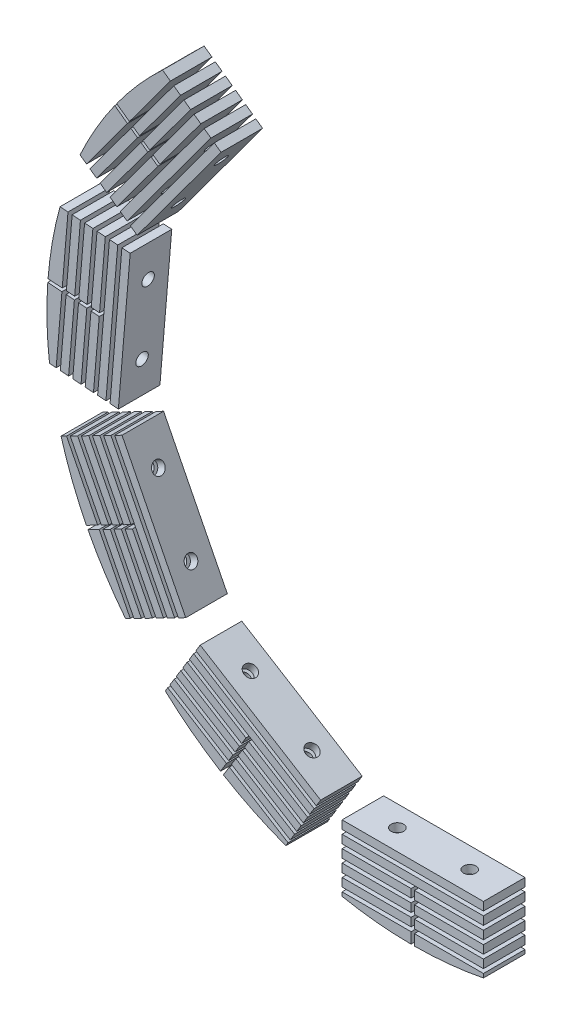
SolidWorks part; units mm, degrees
ref_plane "前视基准面" through (0, 0, 0) normal (0, 0, 1) x (1, 0, 0)
ref_plane "上视基准面" through (0, 0, 0) normal (0, 1, 0) x (1, 0, 0)
ref_plane "右视基准面" through (0, 0, 0) normal (1, 0, 0) x (0, 0, -1)
other "Configuration Table"
sketch "草图1" plane through (0, 0, 0) normal (0, 0, 1) x (1, 0, 0)
  line L0 (-85, -337) -> (-85, -431.7117)
  line L1 (-85, -337) -> (85, -337)
  line L5 (85, -337) -> (85, -431.7117)
  line L18 (-266.8501, -222.677) -> (-129.3172, -322.6005)
  line L19 (-266.8501, -222.677) -> (-322.5202, -299.3004)
  line L20 (-129.3172, -322.6005) -> (-184.9873, -399.2239)
  line L21 (-346.7725, -23.2989) -> (-294.2396, -184.9785)
  line L22 (-346.7725, -23.2989) -> (-436.8487, -52.5665)
  line L23 (-294.2396, -184.9785) -> (-384.3158, -214.2461)
  line L24 (-294.2396, 184.9785) -> (-346.7725, 23.2989)
  line L25 (-294.2396, 184.9785) -> (-384.3158, 214.2461)
  line L26 (-346.7725, 23.2989) -> (-436.8487, 52.5665)
  line L27 (-129.3172, 322.6005) -> (-266.8501, 222.677)
  line L28 (-129.3172, 322.6005) -> (-184.9873, 399.2239)
  line L29 (-266.8501, 222.677) -> (-322.5202, 299.3004)
  line L30 (85, 337) -> (-85, 337)
  line L31 (85, 337) -> (85, 431.7117)
  line L32 (-85, 337) -> (-85, 431.7117)
  line L33 (266.8501, 222.677) -> (129.3172, 322.6005)
  line L34 (266.8501, 222.677) -> (322.5202, 299.3004)
  line L35 (129.3172, 322.6005) -> (184.9873, 399.2239)
  line L36 (346.7725, 23.2989) -> (294.2396, 184.9785)
  line L37 (346.7725, 23.2989) -> (436.8487, 52.5665)
  line L38 (294.2396, 184.9785) -> (384.3158, 214.2461)
  line L39 (294.2396, -184.9785) -> (346.7725, -23.2989)
  line L40 (294.2396, -184.9785) -> (384.3158, -214.2461)
  line L41 (346.7725, -23.2989) -> (436.8487, -52.5665)
  line L42 (129.3172, -322.6005) -> (266.8501, -222.677)
  line L43 (129.3172, -322.6005) -> (184.9873, -399.2239)
  line L44 (266.8501, -222.677) -> (322.5202, -299.3004)
  arc A2 (-85, -431.7117) -> (85, -431.7117) centre (0, 0) ccw
  arc A5 (-322.5202, -299.3004) -> (-184.9873, -399.2239) centre (0, 0) ccw
  arc A6 (-436.8487, -52.5665) -> (-384.3158, -214.2461) centre (0, 0) ccw
  arc A7 (-384.3158, 214.2461) -> (-436.8487, 52.5665) centre (0, 0) ccw
  arc A8 (-184.9873, 399.2239) -> (-322.5202, 299.3004) centre (0, 0) ccw
  arc A9 (85, 431.7117) -> (-85, 431.7117) centre (0, 0) ccw
  arc A10 (322.5202, 299.3004) -> (184.9873, 399.2239) centre (0, 0) ccw
  arc A11 (436.8487, 52.5665) -> (384.3158, 214.2461) centre (0, 0) ccw
  arc A12 (384.3158, -214.2461) -> (436.8487, -52.5665) centre (0, 0) ccw
  arc A13 (184.9873, -399.2239) -> (322.5202, -299.3004) centre (0, 0) ccw
  point P7 (0, -337)
  dimension "D1" = 440
  dimension "D2" = 337
  dimension "D3" = 170
  dimension "D4" = 10
sketch "草图2" plane through (0, 0, 0) normal (0, 0, 1) x (1, 0, 0)
  line L0 (-85, -337) -> (-85, -431.7117)
  line L1 (-85, -337) -> (85, -337) construction
  line L2 (85, -337) -> (85, -431.7117)
  line L3 (0, -299.5672) -> (0, -474.8241) construction
  line L4 (-85, -337) -> (-2, -337)
  line L5 (-2, -337) -> (-2, -439.9955)
  line L6 (2, -337) -> (2, -439.9955)
  line L7 (85, -337) -> (2, -337)
  line L8 (-248.2534, -243.237) -> (-177.4302, -286.5162)
  line L9 (-248.2534, -243.237) -> (-297.6394, -324.0537)
  line L10 (-177.4302, -286.5162) -> (-231.1357, -374.4012)
  line L11 (-174.0171, -288.6019) -> (-227.7225, -376.487)
  line L12 (-103.1939, -331.881) -> (-174.0171, -288.6019)
  line L13 (-103.1939, -331.881) -> (-152.58, -412.6977)
  line L14 (-338.6647, -78.1039) -> (-300.7992, -151.9632)
  line L15 (-338.6647, -78.1039) -> (-422.946, -121.3124)
  line L16 (-300.7992, -151.9632) -> (-392.452, -198.9509)
  line L17 (-298.9744, -155.5227) -> (-390.6271, -202.5104)
  line L18 (-261.1089, -229.3821) -> (-298.9744, -155.5227)
  line L19 (-261.1089, -229.3821) -> (-345.3902, -272.5906)
  line L20 (-329.7056, 109.9464) -> (-335.9082, 27.1784)
  line L21 (-329.7056, 109.9464) -> (-424.1525, 117.0242)
  line L22 (-335.9082, 27.1784) -> (-438.6157, 34.8753)
  line L23 (-336.2071, 23.1896) -> (-438.9146, 30.8865)
  line L24 (-342.4097, -59.5783) -> (-336.2071, 23.1896)
  line L25 (-342.4097, -59.5783) -> (-436.8566, -52.5005)
  line L26 (-224.0049, 265.7363) -> (-272.4556, 198.3455)
  line L27 (-224.0049, 265.7363) -> (-300.9049, 321.0237)
  line L28 (-272.4556, 198.3455) -> (-356.0815, 258.4684)
  line L29 (-274.7906, 195.0977) -> (-358.4165, 255.2207)
  line L30 (-323.2413, 127.7069) -> (-274.7906, 195.0977)
  line L31 (-323.2413, 127.7069) -> (-400.1414, 182.9942)
  arc A0 (-85, -431.7117) -> (85, -431.7117) centre (0, 0) ccw construction
  arc A1 (-85, -431.7117) -> (-2, -439.9955) centre (0, 0) ccw
  arc A2 (85, -431.7117) -> (2, -439.9955) centre (0, 0) cw
  arc A3 (-297.6394, -324.0537) -> (-231.1357, -374.4012) centre (0, 0) ccw
  arc A4 (-152.58, -412.6977) -> (-227.7225, -376.487) centre (0, 0) cw
  arc A5 (-422.946, -121.3124) -> (-392.452, -198.9509) centre (0, 0) ccw
  arc A6 (-345.3902, -272.5906) -> (-390.6271, -202.5104) centre (0, 0) cw
  arc A7 (-424.1525, 117.0242) -> (-438.6157, 34.8753) centre (0, 0) ccw
  arc A8 (-436.8566, -52.5005) -> (-438.9146, 30.8865) centre (0, 0) cw
  arc A9 (-300.9049, 321.0237) -> (-356.0815, 258.4684) centre (0, 0) ccw
  arc A10 (-400.1414, 182.9942) -> (-358.4165, 255.2207) centre (0, 0) cw
  point P2 (0, -387.1957)
  dimension "D1" = 2
  dimension "D3" = 31.429
  dimension "D2" = 5
extrude "凸台-拉伸1" add sketch "草图2" along normal mid plane 50
sketch "草图3" plane through (0, 0, 25) normal (0, 0, 1) x (1, 0, 0)
  line L0 (85, -337) -> (2, -337) construction
  line L1 (-88.6131, -347) -> (106.3869, -347)
  line L2 (-88.6131, -347) -> (-88.6131, -352)
  line L3 (-88.6131, -352) -> (106.3869, -352)
  line L4 (106.3869, -347) -> (106.3869, -352)
  line L5 (-88.6131, -362) -> (106.3869, -362)
  line L6 (-88.6131, -367) -> (106.3869, -367)
  line L7 (-88.6131, -362) -> (-88.6131, -367)
  line L8 (106.3869, -362) -> (106.3869, -367)
  line L9 (-88.6131, -377) -> (106.3869, -377)
  line L10 (-88.6131, -382) -> (106.3869, -382)
  line L11 (-88.6131, -377) -> (-88.6131, -382)
  line L12 (106.3869, -377) -> (106.3869, -382)
  line L13 (-88.6131, -392) -> (106.3869, -392)
  line L14 (-88.6131, -397) -> (106.3869, -397)
  line L15 (-88.6131, -392) -> (-88.6131, -397)
  line L16 (106.3869, -392) -> (106.3869, -397)
  line L17 (-88.6131, -407) -> (106.3869, -407)
  line L18 (-88.6131, -412) -> (106.3869, -412)
  line L19 (-88.6131, -407) -> (-88.6131, -412)
  line L20 (106.3869, -407) -> (106.3869, -412)
  line L21 (-88.6131, -422) -> (106.3869, -422)
  line L22 (-88.6131, -427) -> (106.3869, -427)
  line L23 (-88.6131, -422) -> (-88.6131, -427)
  line L24 (106.3869, -422) -> (106.3869, -427)
  line L231 (-297.2911, -317.7031) -> (-131.2044, -419.8803)
  line L242 (-347.3723, -74.3518) -> (-351.8663, -76.5436) [skipped]
  line L243 (-360.8542, -80.9274) -> (-365.3482, -83.1192) [skipped]
  line L244 (-374.3361, -87.5029) -> (-378.8301, -89.6948) [skipped]
  line L245 (-387.818, -94.0785) -> (-392.312, -96.2703) [skipped]
  line L246 (-401.2999, -100.6541) -> (-405.7939, -102.8459) [skipped]
  line L247 (-414.7819, -107.2296) -> (-419.2758, -109.4215) [skipped]
  line L248 (-332.0417, 120.5654) -> (-352.4248, -73.3664) [skipped]
  line L249 (-332.0417, 120.5654) -> (-337.0143, 121.088) [skipped]
  line L250 (-337.0143, 121.088) -> (-357.3974, -72.8437) [skipped]
  line L251 (-352.4248, -73.3664) -> (-357.3974, -72.8437) [skipped]
  line L252 (-367.3426, -71.7984) -> (-372.3152, -71.2758) [skipped]
  line L253 (-382.2604, -70.2305) -> (-387.233, -69.7079) [skipped]
  line L254 (-397.1783, -68.6626) -> (-402.1509, -68.14) [skipped]
  line L255 (-412.0961, -67.0947) -> (-417.0687, -66.572) [skipped]
  line L256 (-427.0139, -65.5267) -> (-431.9865, -65.0041) [skipped]
  line L257 (-346.9596, 122.1333) -> (-351.9322, 122.656) [skipped]
  line L258 (-361.8774, 123.7012) -> (-366.85, 124.2239) [skipped]
  line L259 (-376.7952, 125.2692) -> (-381.7678, 125.7918) [skipped]
  line L260 (-391.713, 126.8371) -> (-396.6856, 127.3597) [skipped]
  line L261 (-406.6309, 128.405) -> (-411.6035, 128.9277) [skipped]
  line L262 (-346.9596, 122.1333) -> (-367.3426, -71.7984) [skipped]
  line L263 (-351.9322, 122.656) -> (-372.3152, -71.2758) [skipped]
  line L264 (-361.8774, 123.7012) -> (-382.2604, -70.2305) [skipped]
  line L265 (-366.85, 124.2239) -> (-387.233, -69.7079) [skipped]
  line L266 (-376.7952, 125.2692) -> (-397.1783, -68.6626) [skipped]
  line L267 (-381.7678, 125.7918) -> (-402.1509, -68.14) [skipped]
  line L268 (-391.713, 126.8371) -> (-412.0961, -67.0947) [skipped]
  line L269 (-396.6856, 127.3597) -> (-417.0687, -66.572) [skipped]
  line L270 (-406.6309, 128.405) -> (-427.0139, -65.5267) [skipped]
  line L271 (-411.6035, 128.9277) -> (-431.9865, -65.0041) [skipped]
  line L272 (-215.7503, 277.7406) -> (-335.8043, 124.0785) [skipped]
  line L273 (-215.7503, 277.7406) -> (-219.6903, 280.8189) [skipped]
  line L274 (-219.6903, 280.8189) -> (-339.7443, 127.1568) [skipped]
  line L275 (-335.8043, 124.0785) -> (-339.7443, 127.1568) [skipped]
  line L276 (-347.6244, 133.3134) -> (-351.5645, 136.3917) [skipped]
  line L277 (-359.4446, 142.5483) -> (-363.3847, 145.6266) [skipped]
  line L278 (-371.2648, 151.7832) -> (-375.2048, 154.8616) [skipped]
  line L279 (-383.0849, 161.0182) -> (-387.025, 164.0965) [skipped]
  line L280 (-394.9051, 170.2531) -> (-398.8451, 173.3314) [skipped]
  line L281 (-227.5705, 286.9755) -> (-231.5105, 290.0538) [skipped]
  line L282 (-239.3906, 296.2104) -> (-243.3307, 299.2887) [skipped]
  line L283 (-251.2108, 305.4453) -> (-255.1508, 308.5236) [skipped]
  line L284 (-263.0309, 314.6803) -> (-266.971, 317.7586) [skipped]
  line L285 (-274.8511, 323.9152) -> (-278.7912, 326.9935) [skipped]
  line L286 (-227.5705, 286.9755) -> (-347.6244, 133.3134) [skipped]
  line L287 (-231.5105, 290.0538) -> (-351.5645, 136.3917) [skipped]
  line L288 (-239.3906, 296.2104) -> (-359.4446, 142.5483) [skipped]
  line L289 (-243.3307, 299.2887) -> (-363.3847, 145.6266) [skipped]
  line L290 (-251.2108, 305.4453) -> (-371.2648, 151.7832) [skipped]
  line L291 (-255.1508, 308.5236) -> (-375.2048, 154.8616) [skipped]
  line L292 (-263.0309, 314.6803) -> (-383.0849, 161.0182) [skipped]
  line L293 (-266.971, 317.7586) -> (-387.025, 164.0965) [skipped]
  line L294 (-274.8511, 323.9152) -> (-394.9051, 170.2531) [skipped]
  line L295 (-278.7912, 326.9935) -> (-398.8451, 173.3314) [skipped]
  line L296 (-33.8394, 349.4076) -> (-217.0795, 282.7137) [skipped]
  line L297 (-33.8394, 349.4076) -> (-35.5495, 354.1061) [skipped]
  line L298 (-35.5495, 354.1061) -> (-218.7896, 287.4122) [skipped]
  line L299 (-217.0795, 282.7137) -> (-218.7896, 287.4122) [skipped]
  line L300 (-222.2098, 296.8091) -> (-223.9199, 301.5075) [skipped]
  line L301 (-227.3401, 310.9045) -> (-229.0502, 315.6029) [skipped]
  line L302 (-232.4704, 324.9999) -> (-234.1805, 329.6983) [skipped]
  line L303 (-237.6007, 339.0952) -> (-239.3108, 343.7937) [skipped]
  line L304 (-242.731, 353.1906) -> (-244.4411, 357.8891) [skipped]
  line L305 (-38.9697, 363.503) -> (-40.6798, 368.2015) [skipped]
  line L306 (-44.1, 377.5984) -> (-45.8101, 382.2969) [skipped]
  line L307 (-49.2303, 391.6938) -> (-50.9404, 396.3922) [skipped]
  line L308 (-54.3606, 405.7892) -> (-56.0707, 410.4876) [skipped]
  line L309 (-59.4909, 419.8846) -> (-61.201, 424.583) [skipped]
  line L310 (-38.9697, 363.503) -> (-222.2098, 296.8091) [skipped]
  line L311 (-40.6798, 368.2015) -> (-223.9199, 301.5075) [skipped]
  line L312 (-44.1, 377.5984) -> (-227.3401, 310.9045) [skipped]
  line L313 (-45.8101, 382.2969) -> (-229.0502, 315.6029) [skipped]
  line L314 (-49.2303, 391.6938) -> (-232.4704, 324.9999) [skipped]
  line L315 (-50.9404, 396.3922) -> (-234.1805, 329.6983) [skipped]
  line L316 (-54.3606, 405.7892) -> (-237.6007, 339.0952) [skipped]
  line L317 (-56.0707, 410.4876) -> (-239.3108, 343.7937) [skipped]
  line L318 (-59.4909, 419.8846) -> (-242.731, 353.1906) [skipped]
  line L319 (-61.201, 424.583) -> (-244.4411, 357.8891) [skipped]
  line L320 (-115.56, -389.2713) -> (-118.2096, -393.5116) [skipped]
  line L321 (-123.5088, -401.992) -> (-126.1584, -406.2323) [skipped]
  line L322 (-131.4576, -414.7128) -> (-134.1072, -418.953) [skipped]
  line L323 (-107.6112, -376.5506) -> (-110.2608, -380.7908) [skipped]
  line L324 (-91.7136, -351.1092) -> (-94.3632, -355.3494) [skipped]
  line L325 (-99.6624, -363.8299) -> (-102.312, -368.0701) [skipped]
  line L326 (-265.0318, -260.4956) -> (-267.6814, -264.7359) [skipped]
  line L327 (-272.9806, -273.2163) -> (-275.6302, -277.4566) [skipped]
  line L328 (-280.9294, -285.9371) -> (-283.579, -290.1773) [skipped]
  line L329 (-288.8781, -298.6578) -> (-291.5277, -302.898) [skipped]
  line L330 (-296.8269, -311.3785) -> (-299.4765, -315.6188) [skipped]
  line L331 (-265.0318, -260.4956) -> (-99.6624, -363.8299) [skipped]
  line L332 (-267.6814, -264.7359) -> (-102.312, -368.0701) [skipped]
  line L333 (-272.9806, -273.2163) -> (-107.6112, -376.5506) [skipped]
  line L334 (-275.6302, -277.4566) -> (-110.2608, -380.7908) [skipped]
  line L335 (-280.9294, -285.9371) -> (-115.56, -389.2713) [skipped]
  line L336 (-283.579, -290.1773) -> (-118.2096, -393.5116) [skipped]
  line L337 (-288.8781, -298.6578) -> (-123.5088, -401.992) [skipped]
  line L338 (-291.5277, -302.898) -> (-126.1584, -406.2323) [skipped]
  line L339 (-296.8269, -311.3785) -> (-131.4576, -414.7128) [skipped]
  line L340 (-299.4765, -315.6188) -> (-134.1072, -418.953) [skipped]
  line L341 (-257.083, -247.7749) -> (-91.7136, -351.1092) [skipped]
  line L342 (-257.083, -247.7749) -> (-259.7326, -252.0151) [skipped]
  line L343 (-259.7326, -252.0151) -> (-94.3632, -355.3494) [skipped]
  line L344 (-261.8899, -249.6166) -> (-266.3839, -251.8085) [skipped]
  line L345 (-275.3718, -256.1922) -> (-279.8658, -258.3841) [skipped]
  line L346 (-347.3723, -74.3518) -> (-261.8899, -249.6166) [skipped]
  line L347 (-351.8663, -76.5436) -> (-266.3839, -251.8085) [skipped]
  line L348 (-288.8537, -262.7678) -> (-293.3477, -264.9596) [skipped]
  line L349 (-302.3357, -269.3433) -> (-306.8296, -271.5352) [skipped]
  line L350 (-315.8176, -275.9189) -> (-320.3115, -278.1108) [skipped]
  line L351 (-329.2995, -282.4945) -> (-333.7934, -284.6863) [skipped]
  line L352 (-360.8542, -80.9274) -> (-275.3718, -256.1922) [skipped]
  line L353 (-365.3482, -83.1192) -> (-279.8658, -258.3841) [skipped]
  line L354 (-374.3361, -87.5029) -> (-288.8537, -262.7678) [skipped]
  line L355 (-378.8301, -89.6948) -> (-293.3477, -264.9596) [skipped]
  line L356 (-387.818, -94.0785) -> (-302.3357, -269.3433) [skipped]
  line L357 (-392.312, -96.2703) -> (-306.8296, -271.5352) [skipped]
  line L358 (-401.2999, -100.6541) -> (-315.8176, -275.9189) [skipped]
  line L359 (-405.7939, -102.8459) -> (-320.3115, -278.1108) [skipped]
  line L360 (-414.7819, -107.2296) -> (-329.2995, -282.4945) [skipped]
  line L361 (-419.2758, -109.4215) -> (-333.7934, -284.6863) [skipped]
  line L362 (-294.6712, -313.4444) -> (-128.5844, -415.6217)
  line L363 (-289.4313, -304.9272) -> (-123.3446, -407.1044)
  line L364 (-286.8114, -300.6685) -> (-120.7246, -402.8458)
  line L365 (-281.5715, -292.1513) -> (-115.4848, -394.3285)
  line L366 (-278.9516, -287.8926) -> (-112.8649, -390.0699)
  line L367 (-273.7118, -279.3754) -> (-107.625, -381.5526)
  line L368 (-271.0918, -275.1167) -> (-105.0051, -377.294)
  line L369 (-265.852, -266.5995) -> (-99.7652, -368.7767)
  line L370 (-263.232, -262.3408) -> (-97.1453, -364.5181)
  line L371 (-257.9922, -253.8235) -> (-91.9054, -356.0008)
  line L372 (-255.3722, -249.5649) -> (-89.2855, -351.7422)
  line L373 (-89.2855, -351.7422) -> (-91.9054, -356.0008)
  line L374 (-97.1453, -364.5181) -> (-99.7652, -368.7767)
  line L375 (-105.0051, -377.294) -> (-107.625, -381.5526)
  line L376 (-120.7246, -402.8458) -> (-123.3446, -407.1044)
  line L377 (-128.5844, -415.6217) -> (-131.2044, -419.8803)
  line L378 (-112.8649, -390.0699) -> (-115.4848, -394.3285)
  line L379 (-255.3722, -249.5649) -> (-257.9922, -253.8235)
  line L380 (-263.232, -262.3408) -> (-265.852, -266.5995)
  line L381 (-271.0918, -275.1167) -> (-273.7118, -279.3754)
  line L382 (-278.9516, -287.8926) -> (-281.5715, -292.1513)
  line L383 (-286.8114, -300.6685) -> (-289.4313, -304.9272)
  line L384 (-294.6712, -313.4444) -> (-297.2911, -317.7031)
  line L385 (-417.7578, -115.2676) -> (-329.8367, -289.3218)
  line L386 (-413.2949, -113.0132) -> (-325.3737, -287.0674)
  line L387 (-404.369, -108.5044) -> (-316.4479, -282.5586)
  line L388 (-399.9061, -106.25) -> (-311.985, -280.3043)
  line L389 (-390.9802, -101.7412) -> (-303.0591, -275.7955)
  line L390 (-386.5173, -99.4869) -> (-298.5962, -273.5411)
  line L391 (-377.5914, -94.9781) -> (-289.6703, -269.0323)
  line L392 (-373.1285, -92.7237) -> (-285.2074, -266.7779)
  line L393 (-364.2026, -88.2149) -> (-276.2815, -262.2692)
  line L394 (-359.7397, -85.9605) -> (-271.8186, -260.0148)
  line L395 (-350.8139, -81.4518) -> (-262.8927, -255.506)
  line L396 (-346.3509, -79.1974) -> (-258.4298, -253.2516)
  line L397 (-258.4298, -253.2516) -> (-262.8927, -255.506)
  line L398 (-271.8186, -260.0148) -> (-276.2815, -262.2692)
  line L399 (-285.2074, -266.7779) -> (-289.6703, -269.0323)
  line L400 (-311.985, -280.3043) -> (-316.4479, -282.5586)
  line L401 (-325.3737, -287.0674) -> (-329.8367, -289.3218)
  line L402 (-298.5962, -273.5411) -> (-303.0591, -275.7955)
  line L403 (-346.3509, -79.1974) -> (-350.8139, -81.4518)
  line L404 (-359.7397, -85.9605) -> (-364.2026, -88.2149)
  line L405 (-373.1285, -92.7237) -> (-377.5914, -94.9781)
  line L406 (-386.5173, -99.4869) -> (-390.9802, -101.7412)
  line L407 (-399.9061, -106.25) -> (-404.369, -108.5044)
  line L408 (-413.2949, -113.0132) -> (-417.7578, -115.2676)
  line L409 (-414.2891, 120.275) -> (-430.6063, -74.0411)
  line L410 (-409.3067, 119.8566) -> (-425.6239, -74.4595)
  line L411 (-399.3418, 119.0199) -> (-415.6589, -75.2962)
  line L412 (-394.3593, 118.6015) -> (-410.6765, -75.7146)
  line L413 (-384.3944, 117.7647) -> (-400.7115, -76.5514)
  line L414 (-379.4119, 117.3463) -> (-395.7291, -76.9698)
  line L415 (-369.447, 116.5095) -> (-385.7641, -77.8066)
  line L416 (-364.4645, 116.0911) -> (-380.7817, -78.225)
  line L417 (-354.4996, 115.2544) -> (-370.8168, -79.0617)
  line L418 (-349.5171, 114.836) -> (-365.8343, -79.4801)
  line L419 (-339.5522, 113.9992) -> (-355.8694, -80.3169)
  line L420 (-334.5697, 113.5808) -> (-350.8869, -80.7353)
  line L421 (-350.8869, -80.7353) -> (-355.8694, -80.3169)
  line L422 (-365.8343, -79.4801) -> (-370.8168, -79.0617)
  line L423 (-380.7817, -78.225) -> (-385.7641, -77.8066)
  line L424 (-410.6765, -75.7146) -> (-415.6589, -75.2962)
  line L425 (-425.6239, -74.4595) -> (-430.6063, -74.0411)
  line L426 (-395.7291, -76.9698) -> (-400.7115, -76.5514)
  line L427 (-334.5697, 113.5808) -> (-339.5522, 113.9992)
  line L428 (-349.5171, 114.836) -> (-354.4996, 115.2544)
  line L429 (-364.4645, 116.0911) -> (-369.447, 116.5095)
  line L430 (-379.4119, 117.3463) -> (-384.3944, 117.7647)
  line L431 (-394.3593, 118.6015) -> (-399.3418, 119.0199)
  line L432 (-409.3067, 119.8566) -> (-414.2891, 120.275)
  line L433 (-287.9138, 319.0755) -> (-403.6305, 162.1212)
  line L434 (-283.8893, 316.1084) -> (-399.606, 159.1541)
  line L435 (-275.8404, 310.1742) -> (-391.5571, 153.2199)
  line L436 (-271.8159, 307.2071) -> (-387.5326, 150.2528)
  line L437 (-263.767, 301.2729) -> (-379.4837, 144.3186)
  line L438 (-259.7425, 298.3058) -> (-375.4592, 141.3515)
  line L439 (-251.6936, 292.3716) -> (-367.4103, 135.4174)
  line L440 (-247.6691, 289.4046) -> (-363.3858, 132.4503)
  line L441 (-239.6202, 283.4704) -> (-355.3369, 126.5161)
  line L442 (-235.5957, 280.5033) -> (-351.3124, 123.549)
  line L443 (-227.5468, 274.5691) -> (-343.2635, 117.6148)
  line L444 (-223.5223, 271.602) -> (-339.239, 114.6477)
  line L445 (-339.239, 114.6477) -> (-343.2635, 117.6148)
  line L446 (-351.3124, 123.549) -> (-355.3369, 126.5161)
  line L447 (-363.3858, 132.4503) -> (-367.4103, 135.4174)
  line L448 (-387.5326, 150.2528) -> (-391.5571, 153.2199)
  line L449 (-399.606, 159.1541) -> (-403.6305, 162.1212)
  line L450 (-375.4592, 141.3515) -> (-379.4837, 144.3186)
  line L451 (-223.5223, 271.602) -> (-227.5468, 274.5691)
  line L452 (-235.5957, 280.5033) -> (-239.6202, 283.4704)
  line L453 (-247.6691, 289.4046) -> (-251.6936, 292.3716)
  line L454 (-259.7425, 298.3058) -> (-263.767, 301.2729)
  line L455 (-271.8159, 307.2071) -> (-275.8404, 310.1742)
  line L456 (-283.8893, 316.1084) -> (-287.9138, 319.0755)
  line L457 (-76.1079, 422.1803) -> (-256.9087, 349.132)
  line L458 (-74.2349, 417.5444) -> (-255.0357, 344.4961)
  line L459 (-70.4888, 408.2725) -> (-251.2896, 335.2243)
  line L460 (-68.6158, 403.6366) -> (-249.4166, 330.5883)
  line L461 (-64.8697, 394.3648) -> (-245.6705, 321.3165)
  line L462 (-62.9967, 389.7289) -> (-243.7975, 316.6806)
  line L463 (-59.2506, 380.457) -> (-240.0514, 307.4087)
  line L464 (-57.3776, 375.8211) -> (-238.1784, 302.7728)
  line L465 (-53.6315, 366.5493) -> (-234.4323, 293.501)
  line L466 (-51.7585, 361.9134) -> (-232.5593, 288.8651)
  line L467 (-48.0124, 352.6415) -> (-228.8132, 279.5932)
  line L468 (-46.1394, 348.0056) -> (-226.9402, 274.9573)
  line L469 (-226.9402, 274.9573) -> (-228.8132, 279.5932)
  line L470 (-232.5593, 288.8651) -> (-234.4323, 293.501)
  line L471 (-238.1784, 302.7728) -> (-240.0514, 307.4087)
  line L472 (-249.4166, 330.5883) -> (-251.2896, 335.2243)
  line L473 (-255.0357, 344.4961) -> (-256.9087, 349.132)
  line L474 (-243.7975, 316.6806) -> (-245.6705, 321.3165)
  line L475 (-46.1394, 348.0056) -> (-48.0124, 352.6415)
  line L476 (-51.7585, 361.9134) -> (-53.6315, 366.5493)
  line L477 (-57.3776, 375.8211) -> (-59.2506, 380.457)
  line L478 (-62.9967, 389.7289) -> (-64.8697, 394.3648)
  line L479 (-68.6158, 403.6366) -> (-70.4888, 408.2725)
  line L480 (-74.2349, 417.5444) -> (-76.1079, 422.1803)
  line L481 (-85, -337) -> (-85, -431.7117) construction
  point P245 (0.1715, -3.6252)
  dimension "D1" = 10
  dimension "D2" = 5
  dimension "D4" = 25
  dimension "D6" = 195
  dimension "D7" = 6
  dimension "D8" = 31.6
  dimension "D3" = 6
  dimension "D5" = 6
extrude "切除-拉伸2" cut sketch "草图3" against normal blind 50
sketch "草图8" plane through (0, 0, 25) normal (0, 0, 1) x (1, 0, 0)
  line L0 (2, -352) -> (85, -352) construction
  line L1 (-85, -352) -> (-2, -352) construction
  line L2 (-181.5154, -300.8724) -> (-110.8218, -344.3634) construction
  line L3 (-255.616, -255.2854) -> (-184.9223, -298.7764) construction
  line L4 (-310.431, -161.3962) -> (-273.0075, -235.4822) construction
  line L5 (-349.6581, -83.7398) -> (-312.2345, -157.8258) construction
  line L6 (-347.1091, 24.0066) -> (-354.0546, -58.7056) construction
  line L7 (-339.8288, 110.705) -> (-346.7743, 27.9928) construction
  line L8 (-282.207, 200.4298) -> (-331.4643, 133.6188) construction
  line L9 (-230.5758, 270.4605) -> (-279.8331, 203.6496) construction
  line L12 (2, -352) -> (85, -352)
  line L13 (-85, -352) -> (-2, -352)
  line L14 (-181.5154, -300.8724) -> (-110.8218, -344.3634)
  line L15 (-255.616, -255.2854) -> (-184.9223, -298.7764)
  line L16 (-310.431, -161.3962) -> (-273.0075, -235.4822)
  line L17 (-349.6581, -83.7398) -> (-312.2345, -157.8258)
  line L18 (-347.1091, 24.0066) -> (-354.0546, -58.7056)
  line L19 (-339.8288, 110.705) -> (-346.7743, 27.9928)
  line L20 (-282.207, 200.4298) -> (-331.4643, 133.6188)
  line L21 (-230.5758, 270.4605) -> (-279.8331, 203.6496)
  line L26 (-279.8331, 203.6496) -> (-282.207, 200.4298)
  line L27 (-331.4643, 133.6188) -> (-339.8288, 110.705)
  line L28 (-354.0546, -58.7056) -> (-349.6581, -83.7398)
  line L29 (-273.0075, -235.4822) -> (-255.616, -255.2854)
  line L30 (-184.9223, -298.7764) -> (-181.5154, -300.8724)
  line L31 (-110.8218, -344.3634) -> (-85, -352)
  line L32 (-2, -352) -> (2, -352)
  line L33 (85, -352) -> (-230.5758, 270.4605)
  line L34 (-346.7743, 27.9928) -> (-347.1091, 24.0066)
  line L35 (-312.2345, -157.8258) -> (-310.431, -161.3962)
  point P20 (-184.9223, 300.892)
  point P21 (0, 0)
sketch "草图9" plane through (0, -352, 0) normal (0, 1, 0) x (1, 0, 0)
  line L0 (85, 25) -> (85, -25) construction
  line L1 (85, 25) -> (2, 25) construction
  line L2 (0, 0) -> (0, 37.3161) construction
  circle A0 centre (43.5, 0) radius 7.5
  circle A1 centre (-43.5, 0) radius 7.5
  point P4 (85, 0)
  point P7 (43.5, 25)
  dimension "D1" = 15
extrude "切除-拉伸5" cut sketch "草图9" against normal blind 25
sketch "草图10" plane through (-184.1143, -299.2735, 0) normal (0.524, 0.8517, 0) x (0.8517, -0.524, 0)
  line L0 (3.0513, -25) -> (3.0513, 25) construction
  line L1 (86.0517, 25) -> (3.0513, 25) construction
  line L2 (0, 0) -> (0, 77.1762) construction
  line L3 (-0.9917, 25) -> (-83.9913, 25) construction
  line L4 (-83.9913, -25) -> (-83.9913, 25) construction
  circle A0 centre (44.5515, 0) radius 7.5
  circle A2 centre (-42.4915, 0) radius 7.5
  point P5 (3.0513, 0)
  point P8 (44.5515, 25)
  point P15 (-42.4915, 25)
  point P18 (-83.9913, 0)
  dimension "D1" = 15
extrude "切除-拉伸6" cut sketch "草图10" against normal blind 25
sketch "草图11" plane through (-312.2767, -157.7423, 0) normal (0.8926, 0.4509, 0) x (0, 0, -1)
  line L0 (-25, 82.908) -> (25, 82.908) construction
  line L1 (25, 82.908) -> (25, -0.0935) construction
  line L2 (0, 0) -> (42.8973, 0) construction
  line L3 (25, -87.0951) -> (25, -4.0936) construction
  circle A0 centre (0, 41.4072) radius 7.5
  circle A2 centre (0, -45.5943) radius 7.5
  point P4 (0, 82.908)
  point P7 (25, 41.4072)
  point P15 (25, -45.5943)
  dimension "D1" = 15
extrude "切除-拉伸7" cut sketch "草图11" against normal blind 25
sketch "草图12" plane through (-346.6804, 29.1116, 0) normal (0.9965, -0.0837, 0) x (0, 0, -1)
  line L0 (25, -88.1263) -> (25, -5.1229) construction
  line L1 (-25, -5.1229) -> (25, -5.1229) construction
  line L2 (0, 0) -> (56.1965, 0) construction
  line L3 (25, 81.8806) -> (25, -1.1228) construction
  circle A0 centre (0, -46.6246) radius 7.5
  circle A2 centre (0, 40.3789) radius 7.5
  point P4 (25, -46.6246)
  point P7 (0, -5.1229)
  point P16 (25, 40.3789)
  dimension "D1" = 15
extrude "切除-拉伸8" cut sketch "草图12" against normal blind 25
sketch "草图13" plane through (-278.562, 205.3736, 0) normal (0.8049, -0.5934, 0) x (0, 0, -1)
  line L0 (-25, -6.1423) -> (25, -6.1423) construction
  line L1 (25, -89.1482) -> (25, -6.1423) construction
  line L2 (0, 0) -> (55.7093, 0) construction
  line L3 (25, 80.8639) -> (25, -2.142) construction
  line L4 (-25, 80.8639) -> (25, 80.8639) construction
  circle A0 centre (0, -47.6453) radius 7.5
  circle A2 centre (0, 39.361) radius 7.5
  point P4 (0, -6.1423)
  point P7 (25, -47.6453)
  point P15 (25, 39.361)
  point P18 (0, 80.8639)
  dimension "D1" = 15
  dimension "D2" = 15
extrude "切除-拉伸9" cut sketch "草图13" against normal blind 25
sketch "草图15" plane through (0, 0, -25) normal (0, 0, -1) x (-1, 0, 0)
  line L0 (95.8243, -320.0424) -> (108.2146, -340.0969)
  line L1 (108.2146, -340.0969) -> (253.0088, -251.0189)
  line L2 (253.0088, -251.0189) -> (243.9028, -236.2173)
  line L3 (243.9028, -236.2173) -> (95.8243, -320.0424)
  line L4 (275.7732, 200.7306) -> (226.5159, 267.5416) construction
  line L5 (278.147, 197.5108) -> (327.4043, 130.6999) construction
  line L7 (278.147, 197.5108) -> (226.5159, 267.5416)
  line L8 (-91.5506, -313.8503) -> (90.5579, -313.8503)
  line L9 (-91.5506, -313.8503) -> (-91.5506, -350.272)
  line L10 (-91.5506, -350.272) -> (90.5579, -350.272)
  line L11 (90.5579, -313.8503) -> (90.5579, -350.272)
  line L12 (278.147, 197.5108) -> (327.4043, 130.6999)
  line L13 (226.5159, 267.5416) -> (203.8645, 253.8576)
  line L14 (203.8645, 253.8576) -> (290.4352, 110.5552)
  line L15 (290.4352, 110.5552) -> (327.4043, 130.6999)
  line L17 (342.1228, 23.633) -> (349.0684, -59.0793) construction
  line L18 (341.7881, 27.6191) -> (334.8426, 110.3313) construction
  line L19 (341.7881, 27.6191) -> (349.0684, -59.0793)
  line L20 (341.7881, 27.6191) -> (334.8426, 110.3313)
  line L21 (334.8426, 110.3313) -> (320.1305, 109.0959)
  line L22 (320.1305, 109.0959) -> (334.3564, -60.3147)
  line L24 (349.0684, -59.0793) -> (334.3564, -60.3147)
  line L25 (305.9816, -159.1151) -> (268.5581, -233.2011) construction
  line L26 (307.7851, -155.5447) -> (345.2086, -81.4588) construction
  line L27 (305.9816, -159.1151) -> (268.5581, -233.2011)
  line L28 (305.9816, -159.1151) -> (345.2086, -81.4588)
  line L29 (345.2086, -81.4588) -> (319.4253, -68.4347)
  line L30 (319.4253, -68.4347) -> (242.7747, -220.177)
  line L31 (242.7747, -220.177) -> (268.5581, -233.2011)
extrude "切除-拉伸13" cut sketch "草图15" against normal blind 146
sketch "草图16" plane through (0, 0, -25) normal (0, 0, -1) x (-1, 0, 0)
  circle A0 centre (248.2534, -243.237) radius 12.3794
  circle A1 centre (337.5067, -76.937) radius 10.5721
  circle A2 centre (329.7056, 109.9464) radius 6.5348
  circle A3 centre (323.2413, 127.7069) radius 5.1272
extrude "切除-拉伸14" cut sketch "草图16" against normal blind 146
sketch "草图17" plane through (0, 0, -25) normal (0, 0, -1) x (-1, 0, 0)
  line L0 (-2, -352) -> (-2, -362) construction
  line L1 (2, -362) -> (2, -352) construction
  line L2 (2, -377) -> (2, -367) construction
  line L3 (-2, -367) -> (-2, -377) construction
  line L4 (2, -362) -> (2, -352)
  line L5 (2, -377) -> (2, -367)
  line L6 (-2, -367) -> (-2, -377)
  line L7 (-2, -352) -> (-2, -362)
  line L8 (-2, -352) -> (2, -352)
  line L9 (-2, -362) -> (2, -362)
  line L10 (-2, -367) -> (2, -367)
  line L11 (-2, -377) -> (2, -377)
  line L12 (197.9583, -320.1088) -> (192.7439, -311.5758) construction
  line L13 (181.5154, -300.8724) -> (186.7298, -309.4053) construction
  line L14 (190.1367, -307.3094) -> (184.9223, -298.7764) construction
  line L15 (189.337, -313.6718) -> (194.5513, -322.2047) construction
  line L16 (190.1367, -307.3094) -> (184.9223, -298.7764)
  line L17 (181.5154, -300.8724) -> (186.7298, -309.4053)
  line L18 (189.337, -313.6718) -> (194.5513, -322.2047)
  line L19 (197.9583, -320.1088) -> (192.7439, -311.5758)
  line L20 (181.5154, -300.8724) -> (184.9223, -298.7764)
  line L21 (186.7298, -309.4053) -> (190.1367, -307.3094)
  line L22 (189.337, -313.6718) -> (192.7439, -311.5758)
  line L23 (194.5513, -322.2047) -> (197.9583, -320.1088)
  line L24 (323.7793, -168.2395) -> (332.6782, -172.8017) construction
  line L25 (334.4817, -169.2313) -> (325.5829, -164.6691) construction
  line L26 (321.1334, -162.388) -> (312.2345, -157.8258) construction
  line L27 (310.431, -161.3962) -> (319.3299, -165.9584) construction
  line L28 (323.7793, -168.2395) -> (332.6782, -172.8017)
  line L29 (334.4817, -169.2313) -> (325.5829, -164.6691)
  line L30 (321.1334, -162.388) -> (312.2345, -157.8258)
  line L31 (310.431, -161.3962) -> (319.3299, -165.9584)
  line L32 (312.2345, -157.8258) -> (310.431, -161.3962)
  line L33 (321.1334, -162.388) -> (319.3299, -165.9584)
  line L34 (325.5829, -164.6691) -> (323.7793, -168.2395)
  line L35 (334.4817, -169.2313) -> (332.6782, -172.8017)
  line L36 (371.7054, 29.8611) -> (361.733, 29.1137) construction
  line L37 (356.7468, 28.7401) -> (346.7743, 27.9928) construction
  line L38 (362.0677, 25.1276) -> (372.0402, 25.8749) construction
  line L39 (347.1091, 24.0066) -> (357.0815, 24.754) construction
  line L40 (371.7054, 29.8611) -> (361.733, 29.1137)
  line L41 (356.7468, 28.7401) -> (346.7743, 27.9928)
  line L42 (362.0677, 25.1276) -> (372.0402, 25.8749)
  line L43 (347.1091, 24.0066) -> (357.0815, 24.754)
  line L44 (346.7743, 27.9928) -> (347.1091, 24.0066)
  line L45 (356.7468, 28.7401) -> (357.0815, 24.754)
  line L46 (361.733, 29.1137) -> (362.0677, 25.1276)
  line L47 (371.7054, 29.8611) -> (372.0402, 25.8749)
  line L48 (287.9531, 209.4874) -> (279.8331, 203.6496) construction
  line L49 (300.133, 218.2442) -> (292.0131, 212.4064) construction
  line L50 (294.3869, 209.1865) -> (302.5069, 215.0244) construction
  line L51 (282.207, 200.4298) -> (290.3269, 206.2676) construction
  line L52 (287.9531, 209.4874) -> (279.8331, 203.6496)
  line L53 (300.133, 218.2442) -> (292.0131, 212.4064)
  line L54 (294.3869, 209.1865) -> (302.5069, 215.0244)
  line L55 (282.207, 200.4298) -> (290.3269, 206.2676)
  line L56 (279.8331, 203.6496) -> (282.207, 200.4298)
  line L57 (287.9531, 209.4874) -> (290.3269, 206.2676)
  line L58 (292.0131, 212.4064) -> (294.3869, 209.1865)
  line L59 (300.133, 218.2442) -> (302.5069, 215.0244)
extrude "凸台-拉伸2" add sketch "草图17" against normal up to surface (50 mm away) up to face at (-355.5681, -16.9758, 25)
